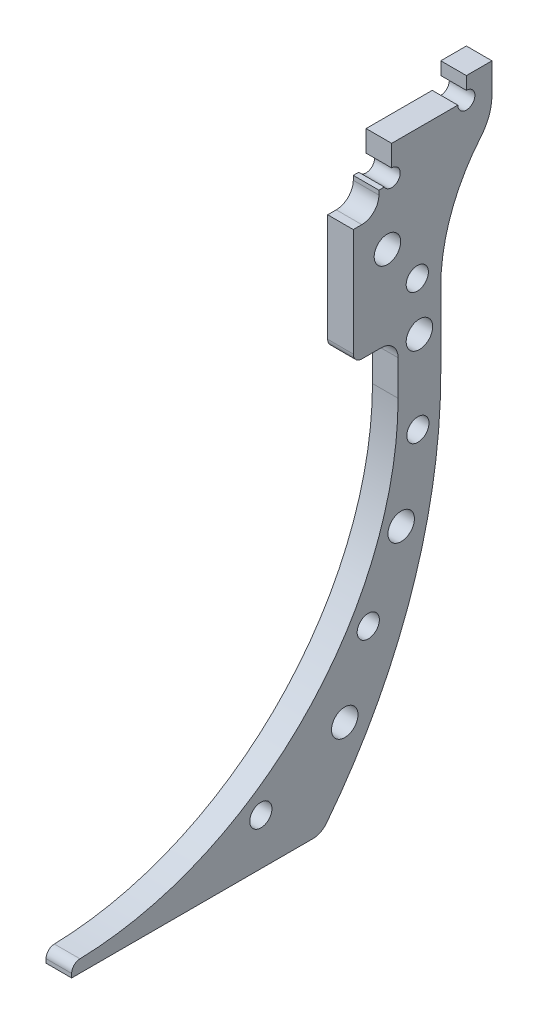
from build123d import *

# Parameters (mm, degrees)
SKETCH_1_R      = 1.55
SKETCH_1_R_2    = 1.3
EXTRUDE_1_DEPTH = 3
SKETCH_2_W      = 0.25
SKETCH_2_H      = 13.633784975
EXTRUDE_2_DEPTH = 3
FILLET_R2_1_R   = 2
FILLET_R1_2_R   = 1


with BuildPart() as part:
    # 草图1 → 凸台-拉伸1 (new body)
    with BuildSketch(Plane(origin=(0, 0, 0), x_dir=(0, 0, -1), z_dir=(1, 0, 0))):
        with BuildLine():
            Line((9.25, 19.75), (9.25, 6.116215025))
            Line((9.25, 6.116215025), (14.25, 6.116215025))
            Line((14.25, 6.116215025), (14.25, 0))
            ThreePointArc((14.25, 0), (3.04683438, -27.04683438), (-24, -38.25))
            Line((-24, -38.25), (-24, -39.7))
            Line((-24, -39.7), (5.238932767, -39.7))
            ThreePointArc((5.238932767, -39.7), (15.644467461, -21.049940647), (19.25, 0))
            Line((19.25, 0), (19.25, 19.75))
            Line((19.25, 19.75), (9.25, 19.75))
        make_face()
        with Locations((13, 15.75)):
            Circle(SKETCH_1_R, mode=Mode.SUBTRACT)
        with Locations((16.75, 5.25)):
            Circle(SKETCH_1_R, mode=Mode.SUBTRACT)
        with Locations((16.5, 11.05)):
            Circle(SKETCH_1_R_2, mode=Mode.SUBTRACT)
        with Locations((-1.828452918, -34.25)):
            Circle(SKETCH_1_R_2, mode=Mode.SUBTRACT)
        with Locations((8, -29.75)):
            Circle(SKETCH_1_R, mode=Mode.SUBTRACT)
        with Locations((10.756717193, -21.368448937)):
            Circle(SKETCH_1_R_2, mode=Mode.SUBTRACT)
        with Locations((14.615659071, -13.170834237)):
            Circle(SKETCH_1_R, mode=Mode.SUBTRACT)
        with Locations((16.57025586, -4.32369512)):
            Circle(SKETCH_1_R_2, mode=Mode.SUBTRACT)
    extrude(amount=EXTRUDE_1_DEPTH)

    # 草图2 → 凸台-拉伸2 (add, through all)
    with BuildSketch(Plane(origin=(3, 0, 0), x_dir=(0, 0, -1), z_dir=(1, 0, 0))):
        with Locations((9.125, 12.933107513)):
            Rectangle(SKETCH_2_W, SKETCH_2_H)
        with BuildLine():
            Line((12, 19.75), (19.25, 19.75))
            Line((19.25, 19.75), (19.25, 8.800075988))
            ThreePointArc((19.25, 8.800075988), (20.460820452, 15.653303833), (23.94667319, 21.676728835))
            ThreePointArc((23.94667319, 21.676728835), (24.913997325, 23.348229273), (25.25, 25.25))
            Line((25.25, 25.25), (25.25, 28.75))
            Line((25.25, 28.75), (22.25, 28.75))
            Line((22.25, 28.75), (22.25, 27.25))
            ThreePointArc((22.25, 27.25), (22.957106781, 25.542893219), (21.25, 26.25))
            Line((21.25, 26.25), (13.5, 26.25))
            Line((13.5, 26.25), (13.5, 23.75))
            ThreePointArc((13.5, 23.75), (14.366025404, 22.25), (12.633974596, 22.25))
            Line((12.633974596, 22.25), (12, 22.25))
            Line((12, 22.25), (12, 19.75))
        make_face()
    extrude(amount=-EXTRUDE_2_DEPTH)

    # R2 圆角1
    fillet_r2_1_edges = [part.edges().sort_by_distance(p)[0] for p in [
        (1.5, -39.7, -5.238932767),
        (1.5, 6.116215025, -14.25),
        (1.5, 19.75, -12),
    ]]
    fillet(fillet_r2_1_edges, radius=FILLET_R2_1_R)

    # R1 圆角2
    fillet_r1_2_edges = [part.edges().sort_by_distance(p)[0] for p in [
        (1.5, -38.25, 24),
        (1.5, 6.116215025, -9),
    ]]
    fillet(fillet_r1_2_edges, radius=FILLET_R1_2_R)


solid = part.part
